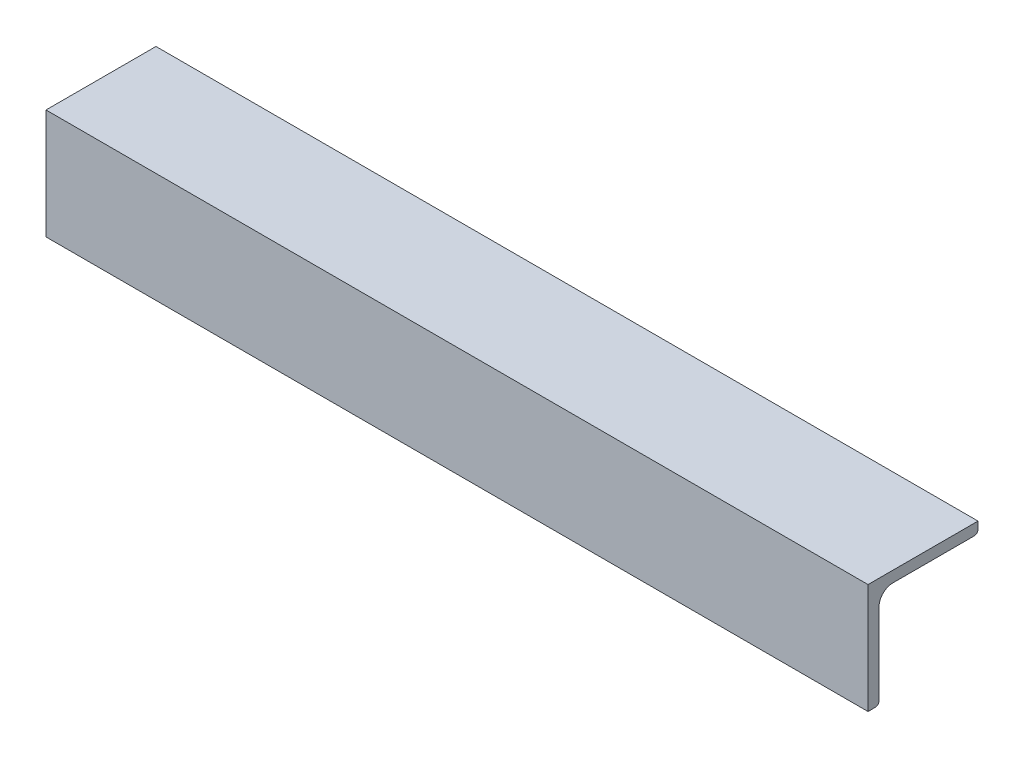
SolidWorks part; units mm, degrees
material "Q235A"
ref_plane "前视基准面" through (0, 0, 0) normal (0, 0, 1) x (1, 0, 0)
ref_plane "上视基准面" through (0, 0, 0) normal (0, 1, 0) x (1, 0, 0)
ref_plane "右视基准面" through (0, 0, 0) normal (1, 0, 0) x (0, 0, -1)
sketch "草图2" plane through (0, 0, 0) normal (0, 1, 0) x (1, 0, 0)
  line L0 (0, 0) -> (299, 0)
  dimension "D1" = 299
ref_plane "基准面1" through (0, 0, 0) normal (1, 0, 0) x (0, 0, -1)
other "等边角钢 4X4(1)"
ref_plane "基准面2" through (0, 0, 0) normal (1, 0, 0) x (0, 0, -1)
sketch "Sketch13" plane through (0, 0, 0) normal (1, 0, 0) x (0, 0, -1)
  line L0 (40, 0) -> (0, 0)
  line L1 (0, 0) -> (0, -40)
  line L2 (38.6667, -4) -> (9, -4)
  line L3 (4, -9) -> (4, -38.6667)
  line L4 (40, 0) -> (40, -2.6667)
  line L5 (0, -40) -> (2.6667, -40)
  arc A0 (40, -2.6667) -> (38.6667, -4) centre (38.6667, -2.6667) cw
  arc A1 (2.6667, -40) -> (4, -38.6667) centre (2.6667, -38.6667) ccw
  arc A2 (9, -4) -> (4, -9) centre (9, -9) ccw
  point P2 (20, 0)
  point P13 (0, -20)
  point P15 (0, 0)
  dimension "r1" = 1.3333
  dimension "r" = 5
  dimension "b" = 40
  dimension "d" = 4
